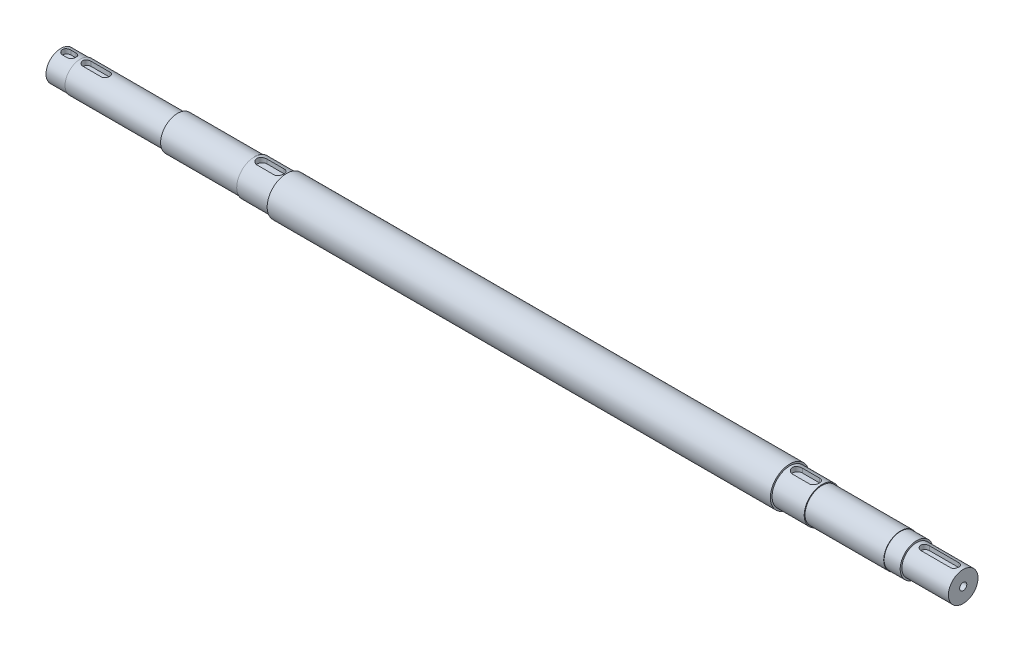
from build123d import *

# Parameters (mm, degrees)
SKETCH_1_R              = 23
EXTRUDE_1_DEPTH         = 595
SKETCH_2_R              = 21
EXTRUDE_2_DEPTH         = 38
SKETCH_3_R              = 20
EXTRUDE_3_DEPTH         = 91
SKETCH_4_R              = 18
EXTRUDE_4_DEPTH         = 115
SKETCH_5_R              = 17.5
EXTRUDE_5_DEPTH         = 23
EXTRUDE_START           = 38
SKETCH_7_R              = 21
EXTRUDE_6_DEPTH         = 38
CUT_EXTRUDE_2_DEPTH     = 5.88
CUT_EXTRUDE_3_DEPTH     = 6.03
EXTRUDE_START_2         = 93
SKETCH_10_R             = 20
EXTRUDE_7_DEPTH         = 93
SKETCH_11_R             = 19.5
EXTRUDE_8_DEPTH         = 19
EXTRUDE_START_3         = 55
SKETCH_12_R             = 17.5
EXTRUDE_9_DEPTH         = 55
CUT_EXTRUDE_4_DEPTH     = 5.73
HOLE_WIZARD_M10_1_D     = 8.5
HOLE_WIZARD_M10_1_DEPTH = 15
HOLE_WIZARD_M10_1_TIP   = 2.553657631
HOLE_WIZARD_M10_2_D     = 8.5
HOLE_WIZARD_M10_2_DEPTH = 15
HOLE_WIZARD_M10_2_TIP   = 2.553657631


with BuildPart() as part:
    # 草图1 → 凸台-拉伸1 (new body)
    with BuildSketch(Plane(origin=(0, 0, 0), x_dir=(0, 0, -1), z_dir=(1, 0, 0))):
        Circle(SKETCH_1_R)
    extrude(amount=EXTRUDE_1_DEPTH)

    # 草图2 → 凸台-拉伸2 (add)
    with BuildSketch(Plane.ZY):
        with Locations(Location((0, 0, 0), (0, 0, 180))):
            Circle(SKETCH_2_R)
    extrude(amount=EXTRUDE_2_DEPTH)

    # 草图3 → 凸台-拉伸3 (add)
    with BuildSketch(Plane.ZY.offset(38)):
        Circle(SKETCH_3_R)
    extrude(amount=EXTRUDE_3_DEPTH)

    # 草图4 → 凸台-拉伸4 (add)
    with BuildSketch(Plane.ZY.offset(129)):
        Circle(SKETCH_4_R)
    extrude(amount=EXTRUDE_4_DEPTH)

    # 草图5 → 凸台-拉伸5 (add)
    with BuildSketch(Plane.ZY.offset(244)):
        Circle(SKETCH_5_R)
    extrude(amount=EXTRUDE_5_DEPTH)

    # 草图7 → 凸台-拉伸6 (add)
    with BuildSketch(Plane(origin=(595, 0, 0), x_dir=(0, 0, -1), z_dir=(1, 0, 0)).offset(EXTRUDE_START)):
        Circle(SKETCH_7_R)
    extrude(amount=-EXTRUDE_6_DEPTH)

    # 草图6 → 切除-拉伸2 (cut)
    with BuildSketch(Plane(origin=(0, 21, 0), x_dir=(1, 0, 0), z_dir=(0, 1, 0))):
        with BuildLine():
            Line((-9, -6), (-29, -6))
            ThreePointArc((-29, -6), (-35, 0), (-29, 6))
            Line((-29, 6), (-9, 6))
            ThreePointArc((-9, 6), (-3, 0), (-9, -6))
        make_face()
        with BuildLine():
            Line((604, 6), (624, 6))
            ThreePointArc((624, 6), (630, 0), (624, -6))
            Line((624, -6), (604, -6))
            ThreePointArc((604, -6), (598, 0), (604, 6))
        make_face()
    extrude(amount=-CUT_EXTRUDE_2_DEPTH, mode=Mode.SUBTRACT)

    # 草图9 → 切除-拉伸3 (cut)
    with BuildSketch(Plane(origin=(0, 18, 0), x_dir=(1, 0, 0), z_dir=(0, 1, 0))):
        with BuildLine():
            Line((-236, 5), (-214, 5))
            ThreePointArc((-214, 5), (-209, 0), (-214, -5))
            Line((-214, -5), (-236, -5))
            ThreePointArc((-236, -5), (-241, 0), (-236, 5))
        make_face()
    cut_extrude_3 = extrude(amount=-CUT_EXTRUDE_3_DEPTH, mode=Mode.SUBTRACT)

    # 草图10 → 凸台-拉伸7 (add)
    with BuildSketch(Plane(origin=(633, 0, 0), x_dir=(0, 0, -1), z_dir=(1, 0, 0)).offset(EXTRUDE_START_2)):
        with Locations(Location((0, 0, 0), (0, 0, 180))):
            Circle(SKETCH_10_R)
    extrude(amount=-EXTRUDE_7_DEPTH)

    # 草图11 → 凸台-拉伸8 (add)
    with BuildSketch(Plane(origin=(726, 0, 0), x_dir=(0, 0, -1), z_dir=(1, 0, 0))):
        Circle(SKETCH_11_R)
    extrude(amount=EXTRUDE_8_DEPTH)

    # 草图12 → 凸台-拉伸9 (add)
    with BuildSketch(Plane(origin=(745, 0, 0), x_dir=(0, 0, -1), z_dir=(1, 0, 0)).offset(EXTRUDE_START_3)):
        with Locations(Location((0, 0, 0), (0, 0, 180))):
            Circle(SKETCH_12_R)
    extrude(amount=-EXTRUDE_9_DEPTH)

    # 草图13 → 切除-拉伸4 (cut)
    with BuildSketch(Plane(origin=(0, 17.5, 0), x_dir=(1, 0, 0), z_dir=(0, 1, 0))):
        with BuildLine():
            Line((-254, -5), (-260, -5))
            ThreePointArc((-260, -5), (-265, 0), (-260, 5))
            Line((-260, 5), (-254, 5))
            ThreePointArc((-254, 5), (-249, 0), (-254, -5))
        make_face()
        with BuildLine():
            Line((790, -5), (755, -5))
            ThreePointArc((755, -5), (750, 0), (755, 5))
            Line((755, 5), (790, 5))
            ThreePointArc((790, 5), (795, 0), (790, -5))
        make_face()
    extrude(amount=-CUT_EXTRUDE_4_DEPTH, mode=Mode.SUBTRACT)

    # M10 螺纹孔1
    with Locations(Plane.ZY.offset(267)):
        with Locations((0, 0)):
            Hole(HOLE_WIZARD_M10_1_D / 2, depth=HOLE_WIZARD_M10_1_DEPTH)
            with Locations((0, 0, -(HOLE_WIZARD_M10_1_DEPTH + HOLE_WIZARD_M10_1_TIP / 2))):  # 118° drill point
                Cone(0, HOLE_WIZARD_M10_1_D / 2, HOLE_WIZARD_M10_1_TIP, mode=Mode.SUBTRACT)

    # M10 螺纹孔2
    with Locations(Plane(origin=(800, 0, 0), x_dir=(0, 0, -1), z_dir=(1, 0, 0))):
        with Locations((0, 0)):
            Hole(HOLE_WIZARD_M10_2_D / 2, depth=HOLE_WIZARD_M10_2_DEPTH)
            with Locations((0, 0, -(HOLE_WIZARD_M10_2_DEPTH + HOLE_WIZARD_M10_2_TIP / 2))):  # 118° drill point
                Cone(0, HOLE_WIZARD_M10_2_D / 2, HOLE_WIZARD_M10_2_TIP, mode=Mode.SUBTRACT)

    # 镜向1: 切除-拉伸3 across plane
    add(cut_extrude_3.mirror(Plane.ZX), mode=Mode.SUBTRACT)


solid = part.part
